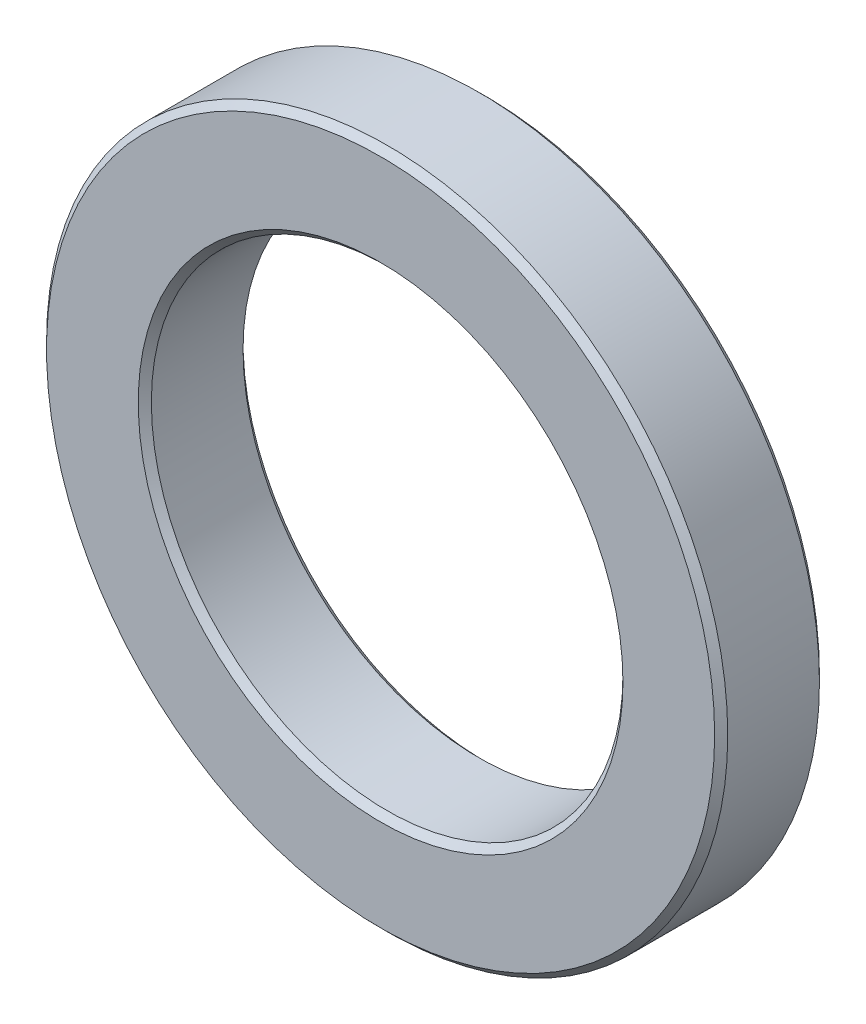
from build123d import *

# Parameters (mm, degrees)
SKETCH1_R           = 26
SKETCH1_R_2         = 18
BOSS_EXTRUDE1_DEPTH = 8
CHAMFER1_SIZE       = 0.5


with BuildPart() as part:
    # Sketch1 → Boss-Extrude1 (new body)
    with BuildSketch(Plane.XY):
        Circle(SKETCH1_R)
        Circle(SKETCH1_R_2, mode=Mode.SUBTRACT)
    extrude(amount=BOSS_EXTRUDE1_DEPTH)

    # Chamfer1
    chamfer1_edges = [part.edges().sort_by_distance(p)[0] for p in [
        (-26, 0, 0),
        (-26, 0, 8),
        (-18, 0, 0),
        (-18, 0, 8),
    ]]
    chamfer(chamfer1_edges, length=CHAMFER1_SIZE)


solid = part.part
